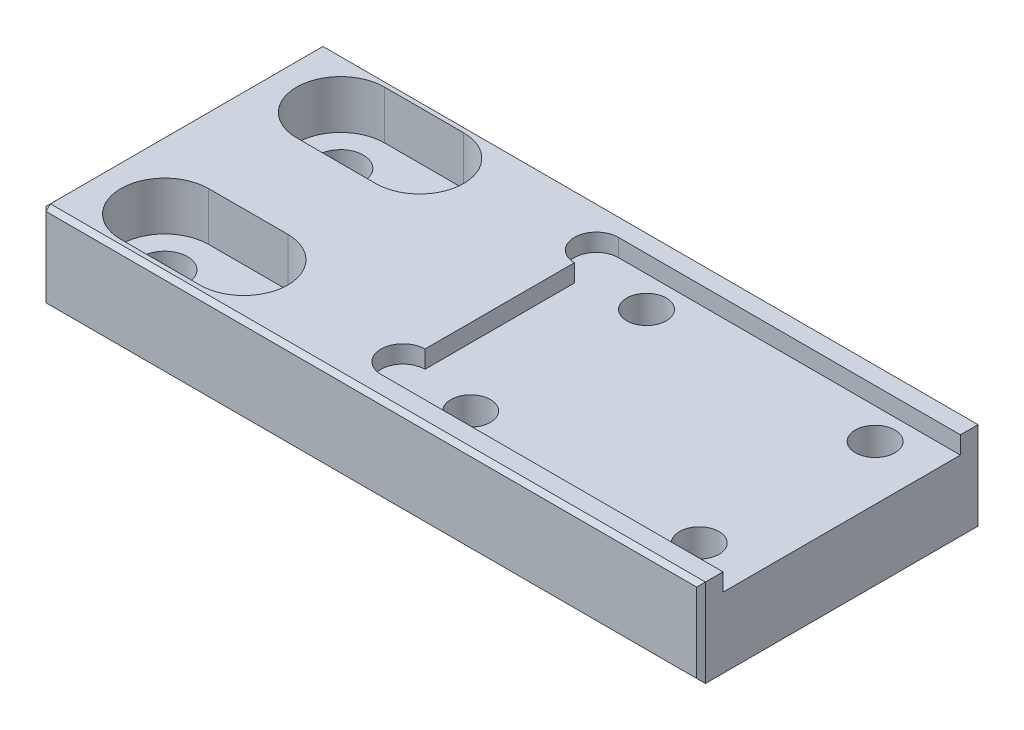
from build123d import *

# Parameters (mm, degrees)
SKETCH1_W                                            = 75
SKETCH1_H                                            = 32
EXTRUDE1_DEPTH                                       = 10
SKETCH2_W                                            = 38.9
SKETCH2_H                                            = 27
EXTRUDE2_DEPTH                                       = 2
CBORE_FOR_M4_HEXAGON_SOCKET_HEAD_CAP_SCR_D           = 4.5
CBORE_FOR_M4_HEXAGON_SOCKET_HEAD_CAP_SCR_CBORE_D     = 8
CBORE_FOR_M4_HEXAGON_SOCKET_HEAD_CAP_SCR_CBORE_DEPTH = 4.6
CBORE_FOR_M5_HEXAGON_SOCKET_HEAD_CAP_SCR_D           = 5.2
CBORE_FOR_M5_HEXAGON_SOCKET_HEAD_CAP_SCR_CBORE_D     = 10
CBORE_FOR_M5_HEXAGON_SOCKET_HEAD_CAP_SCR_CBORE_DEPTH = 5.5
EXTRUDE4_START                                       = 10
EXTRUDE4_DEPTH                                       = 10
SKETCH11_R                                           = 2.5
EXTRUDE6_DEPTH                                       = 2
CHAMFER1_SIZE                                        = 0.5


with BuildPart() as part:
    # Sketch1 → Extrude1 (new body)
    with BuildSketch(Plane(origin=(0, 0, 0), x_dir=(1, 0, 0), z_dir=(0, 1, 0))):
        Rectangle(SKETCH1_W, SKETCH1_H)
    extrude(amount=EXTRUDE1_DEPTH)

    # Sketch2 → Extrude2 (cut)
    with BuildSketch(Plane(origin=(0, 10, 0), x_dir=(1, 0, 0), z_dir=(0, 1, 0))):
        with Locations((18.05, 0)):
            Rectangle(SKETCH2_W, SKETCH2_H)
    extrude(amount=-EXTRUDE2_DEPTH, mode=Mode.SUBTRACT)

    # CBORE for M4 Hexagon socket head cap screws1 (through all)
    with Locations(Plane(origin=(0, 0, 0), x_dir=(-1, 0, 0), z_dir=(0, -1, 0))):
        with Locations((-31.3, -10), (-31.3, 10), (-5.3, 10), (-5.3, -10)):
            CounterBoreHole(CBORE_FOR_M4_HEXAGON_SOCKET_HEAD_CAP_SCR_D / 2, CBORE_FOR_M4_HEXAGON_SOCKET_HEAD_CAP_SCR_CBORE_D / 2, CBORE_FOR_M4_HEXAGON_SOCKET_HEAD_CAP_SCR_CBORE_DEPTH)

    # CBORE for M5 Hexagon socket head cap screws1 (through all)
    with Locations(Plane(origin=(0, 10, 0), x_dir=(1, 0, 0), z_dir=(0, 1, 0))):
        with Locations((-29.5, 10), (-20.5, 10), (-20.5, -10), (-29.5, -10)):
            CounterBoreHole(CBORE_FOR_M5_HEXAGON_SOCKET_HEAD_CAP_SCR_D / 2, CBORE_FOR_M5_HEXAGON_SOCKET_HEAD_CAP_SCR_CBORE_D / 2, CBORE_FOR_M5_HEXAGON_SOCKET_HEAD_CAP_SCR_CBORE_DEPTH)

    # Sketch10 → Extrude4 (cut)
    with BuildSketch(Plane(origin=(0, 4.5, 0), x_dir=(1, 0, 0), z_dir=(0, 1, 0)).offset(EXTRUDE4_START)):
        with BuildLine():
            Line((-29.5, 15), (-20.5, 15))
            ThreePointArc((-20.5, 15), (-15.5, 10), (-20.5, 5))
            Line((-20.5, 5), (-29.5, 5))
            ThreePointArc((-29.5, 5), (-34.5, 10), (-29.5, 15))
        make_face()
        with BuildLine():
            Line((-29.5, -5), (-20.5, -5))
            ThreePointArc((-20.5, -5), (-15.5, -10), (-20.5, -15))
            Line((-20.5, -15), (-29.5, -15))
            ThreePointArc((-29.5, -15), (-34.5, -10), (-29.5, -5))
        make_face()
    extrude(amount=-EXTRUDE4_DEPTH, mode=Mode.SUBTRACT)

    # Sketch11 → Extrude6 (cut)
    with BuildSketch(Plane(origin=(0, 10, 0), x_dir=(1, 0, 0), z_dir=(0, 1, 0))):
        with Locations((-1.4, 11)):
            Circle(SKETCH11_R)
        with Locations((-1.4, -11)):
            Circle(SKETCH11_R)
    extrude(amount=-EXTRUDE6_DEPTH, mode=Mode.SUBTRACT)

    # Chamfer1
    chamfer1_edges = [part.edges().sort_by_distance(p)[0] for p in [
        (0, 10, -16),
        (-37.5, 10, 0),
        (0, 0, -16),
        (0, 0, 16),
        (0, 10, 16),
        (-37.5, 5, -16),
        (37.5, 5, -16),
        (37.5, 5, 16),
        (-37.5, 5, 16),
    ]]
    chamfer(chamfer1_edges, length=CHAMFER1_SIZE)


solid = part.part
